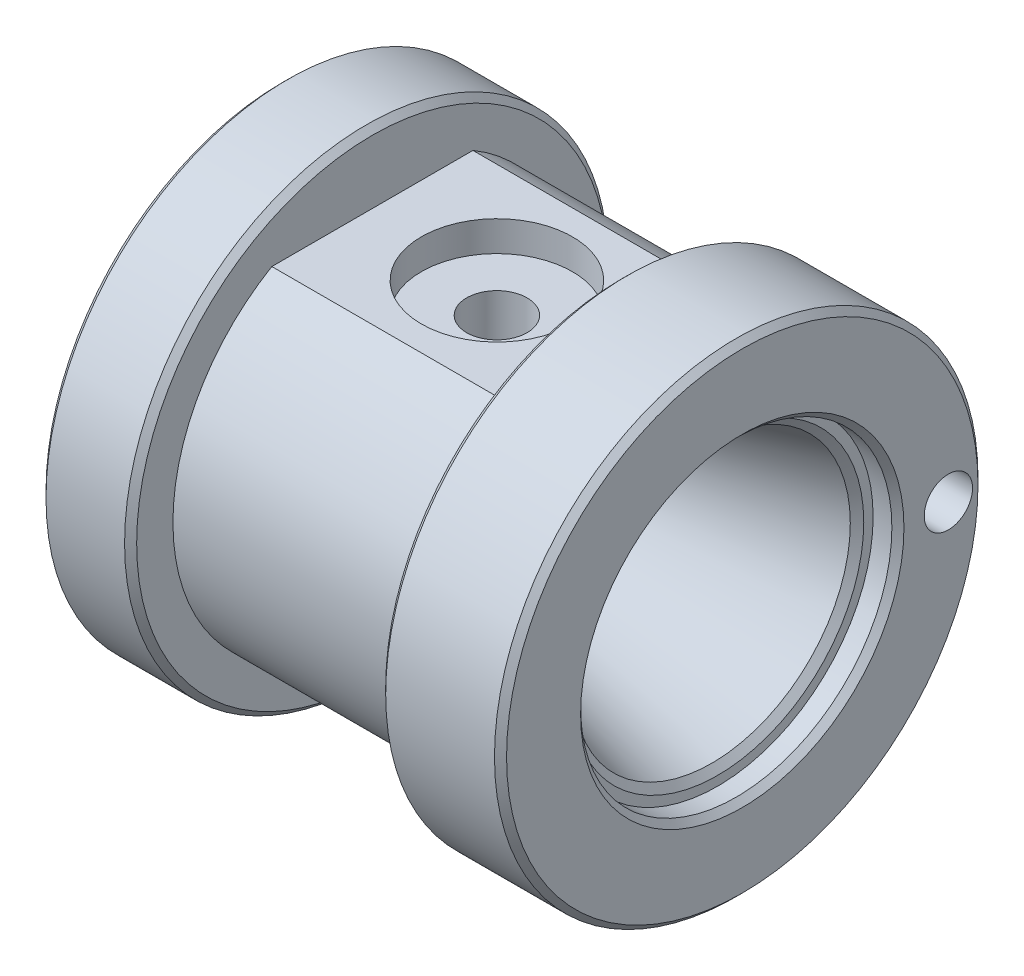
from build123d import *

# Parameters (mm, degrees)
CHAMFER1_SIZE           = 1
CUT_EXTRUDE1_DEPTH      = 95.902265516
CUT_EXTRUDE1_DEPTH_BACK = 95.902265516
SKETCH2_W               = 41.2
SKETCH2_H               = 27.770788335
SKETCH2_H_2             = 30.82392473
SKETCH3_R               = 12.5
CUT_EXTRUDE2_DEPTH      = 5
SKETCH4_R               = 5
CUT_EXTRUDE3_DEPTH      = 19
SKETCH5_R               = 4
CUT_EXTRUDE4_DEPTH      = 10
SKETCH6_R               = 4
CUT_EXTRUDE5_DEPTH      = 13


with BuildPart() as part:
    # Sketch1 → Revolve1 (revolve)
    with BuildSketch(Plane.XY, mode=Mode.PRIVATE) as revolve1_sk:
        with BuildLine():
            Line((0, 26.75), (0, 40))
            Line((0, 40), (-20, 40))
            Line((-20, 40), (-20, 33))
            Line((-20, 33), (-61.2, 33))
            Line((-61.2, 33), (-61.2, 40))
            Line((-61.2, 40), (-76.2, 40))
            Line((-76.2, 40), (-76.2, 26))
            Line((-76.2, 26), (-75.2, 25))
            Line((-75.2, 25), (-65.7, 25))
            Line((-65.7, 25), (-65.7, 20.741987874))
            ThreePointArc((-65.7, 20.741987874), (-58.03253481, 17.787808996), (-52.2, 12))
            Line((-52.2, 12), (-45.1, 12))
            Line((-45.1, 12), (-44.1, 13))
            Line((-44.1, 13), (-44.1, 14.65))
            Line((-44.1, 14.65), (-36, 14.65))
            Line((-36, 14.65), (-5.065925826, 22.938760193))
            Line((-5.065925826, 22.938760193), (-4.1, 24.197579239))
            Line((-4.1, 24.197579239), (-4.1, 25.75))
            Line((-4.1, 25.75), (-1, 25.75))
            Line((-1, 25.75), (0, 26.75))
        make_face()
    revolve(revolve1_sk.sketch.rotate(Axis((23.528076115, 0, 0), (-1, 0, 0)), 90), axis=Axis((23.528076115, 0, 0), (-1, 0, 0)))

    # Chamfer1
    chamfer1_edges = [part.edges().sort_by_distance(p)[0] for p in [
        (0, 0, 40),
        (-20, 0, 40),
        (-61.2, 0, 40),
        (-76.2, 0, 40),
    ]]
    chamfer(chamfer1_edges, length=CHAMFER1_SIZE)

    # Sketch2 → Cut-Extrude1 (cut, two sides: drawn at the far end of the back side and taken through both)
    with BuildSketch(Plane.XY.offset(-CUT_EXTRUDE1_DEPTH_BACK)):
        with Locations((-40.6, 42.385394168)):
            Rectangle(SKETCH2_W, SKETCH2_H)
        with Locations((-40.6, -43.911962365)):
            Rectangle(SKETCH2_W, SKETCH2_H_2)
    extrude(amount=CUT_EXTRUDE1_DEPTH + CUT_EXTRUDE1_DEPTH_BACK, mode=Mode.SUBTRACT)

    # Sketch3 → Cut-Extrude2 (cut)
    with BuildSketch(Plane(origin=(0, 28.5, 0), x_dir=(1, 0, 0), z_dir=(0, 1, 0))):
        with Locations(Location((-40.6, 0, 0), (0, 0, 270))):
            Circle(SKETCH3_R)
    cut_extrude2 = extrude(amount=-CUT_EXTRUDE2_DEPTH, mode=Mode.SUBTRACT)

    # Sketch4 → Cut-Extrude3 (cut)
    with BuildSketch(Plane(origin=(0, 23.5, 0), x_dir=(1, 0, 0), z_dir=(0, 1, 0))):
        with Locations(Location((-40.6, 0, 0), (0, 0, 270))):
            Circle(SKETCH4_R)
    cut_extrude3 = extrude(amount=-CUT_EXTRUDE3_DEPTH, mode=Mode.SUBTRACT)

    # Mirror1: Cut-Extrude2, Cut-Extrude3 across plane
    add(cut_extrude2.mirror(Plane.ZX), mode=Mode.SUBTRACT)
    add(cut_extrude3.mirror(Plane.ZX), mode=Mode.SUBTRACT)

    # Sketch5 → Cut-Extrude4 (cut)
    with BuildSketch(Plane.ZY.offset(76.2)):
        with Locations((-34.097701423, 0)):
            Circle(SKETCH5_R)
    extrude(amount=-CUT_EXTRUDE4_DEPTH, mode=Mode.SUBTRACT)

    # Sketch6 → Cut-Extrude5 (cut)
    with BuildSketch(Plane(origin=(0, 0, 0), x_dir=(0, 0, -1), z_dir=(1, 0, 0))):
        with Locations((34.1, 0)):
            Circle(SKETCH6_R)
    extrude(amount=-CUT_EXTRUDE5_DEPTH, mode=Mode.SUBTRACT)


solid = part.part
